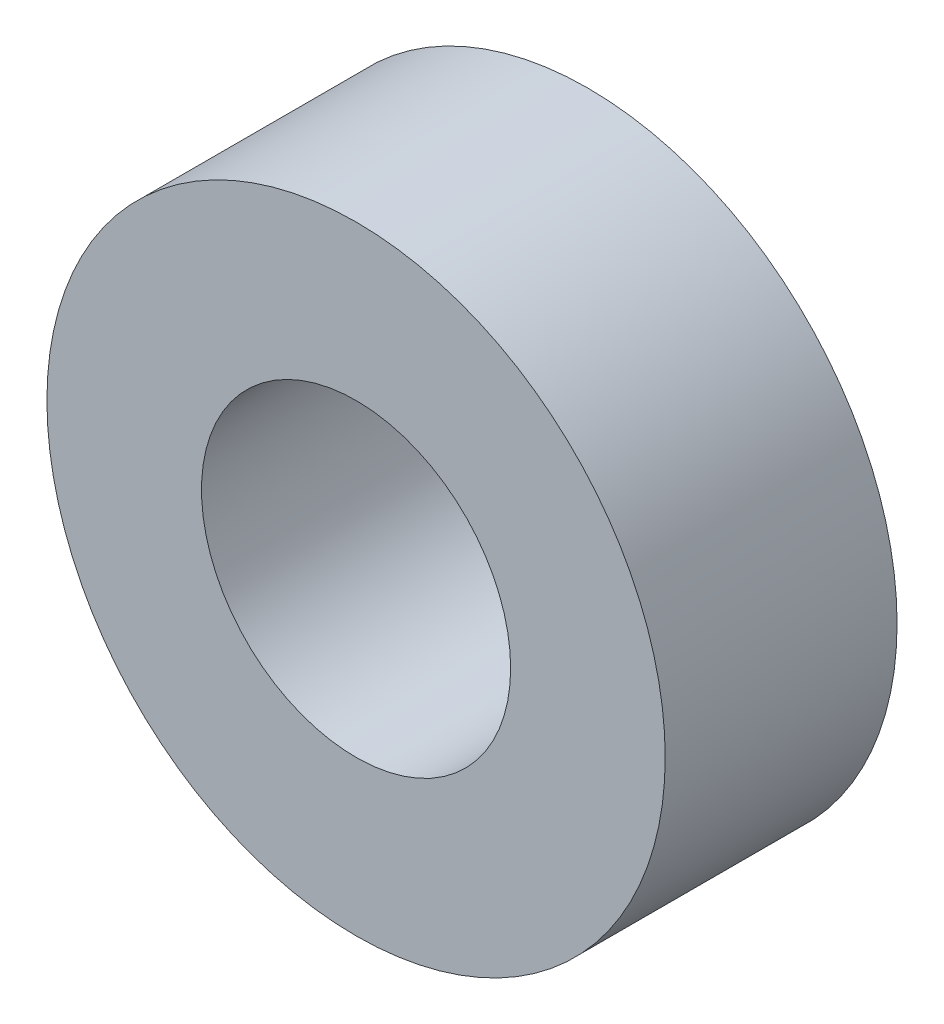
SolidWorks part; units mm, degrees
ref_plane "前视基准面" through (0, 0, 0) normal (0, 0, 1) x (1, 0, 0)
ref_plane "上视基准面" through (0, 0, 0) normal (0, 1, 0) x (1, 0, 0)
ref_plane "右视基准面" through (0, 0, 0) normal (1, 0, 0) x (0, 0, -1)
sketch "草图1" plane through (0, 0, 0) normal (0, 0, 1) x (1, 0, 0)
  circle A0 centre (0, 0) radius 10
  circle A1 centre (0, 0) radius 20
  dimension "D1" = 20
  dimension "D2" = 40
extrude "凸台-拉伸1" add sketch "草图1" along normal mid plane 15
